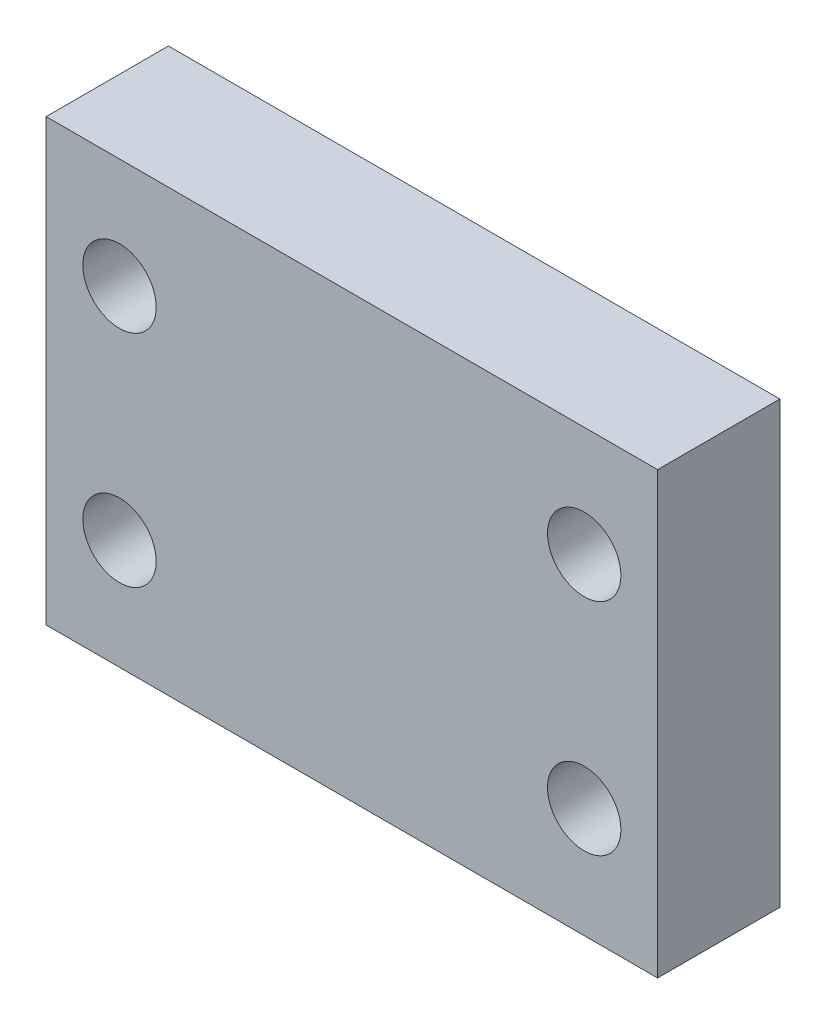
SolidWorks part; units mm, degrees
ref_plane "Front Plane" through (0, 0, 0) normal (0, 0, 1) x (1, 0, 0)
ref_plane "Top Plane" through (0, 0, 0) normal (0, 1, 0) x (1, 0, 0)
ref_plane "Right Plane" through (0, 0, 0) normal (1, 0, 0) x (0, 0, -1)
sketch "Sketch1" plane through (0, 0, 0) normal (0, 0, 1) x (1, 0, 0)
  line L1 (-12.5, -9) -> (12.5, -9)
  line L2 (-12.5, -9) -> (-12.5, 9)
  line L3 (-12.5, 9) -> (12.5, 9)
  line L4 (12.5, -9) -> (12.5, 9)
  line L5 (-12.5, -9) -> (12.5, 9) construction
  line L6 (-12.5, 9) -> (12.5, -9) construction
  circle A0 centre (-9.5, 4.5) radius 1.5
  circle A1 centre (9.5, 4.5) radius 1.5
  circle A2 centre (9.5, -4.5) radius 1.5
  circle A3 centre (-9.5, -4.5) radius 1.5
  point P0 (0, 0)
  dimension "D2" = 3
  dimension "D3" = 3
  dimension "D8" = 3
  dimension "D9" = 3
  dimension "D10" = 19
  dimension "D13" = 3
  dimension "D1" = 18
  dimension "D4" = 4.5
  dimension "D5" = 4.5
  dimension "D6" = 4.5
  dimension "D7" = 9
  dimension "D11" = 25
  dimension "D12" = 3
  dimension "D14" = 19
extrude "Boss-Extrude1" add sketch "Sketch1" along normal blind 5
